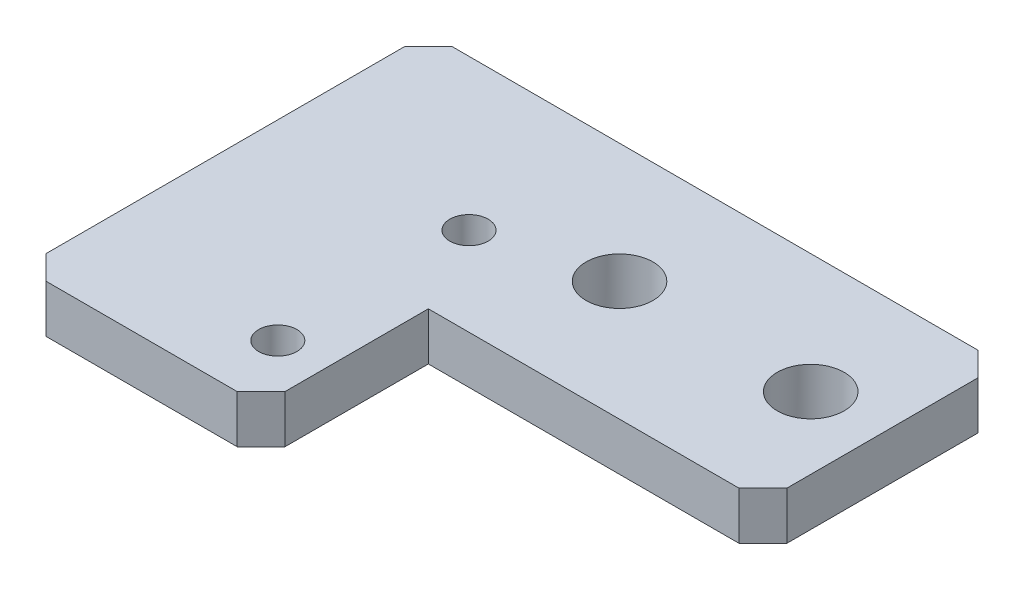
SolidWorks part; units mm, degrees
ref_plane "Front Plane" through (0, 0, 0) normal (0, 0, 1) x (1, 0, 0)
ref_plane "Top Plane" through (0, 0, 0) normal (0, 1, 0) x (1, 0, 0)
ref_plane "Right Plane" through (0, 0, 0) normal (1, 0, 0) x (0, 0, -1)
sketch "Sketch1" plane through (0, 0, 0) normal (0, 1, 0) x (1, 0, 0)
  line L1 (0, 0) -> (10, 0)
  line L2 (0, 0) -> (0, 17)
  line L3 (0, 17) -> (10, 17)
  line L4 (10, 0) -> (10, 17)
  dimension "D1" = 10
  dimension "D2" = 17
extrude "Boss-Extrude1" add sketch "Sketch1" along normal blind 2
sketch "Sketch2" plane through (0, 2, 0) normal (0, 1, 0) x (1, 0, 0)
  line L1 (10, 17) -> (24, 17)
  line L2 (10, 17) -> (10, 7)
  line L3 (10, 7) -> (24, 7)
  line L4 (24, 17) -> (24, 7)
  dimension "D1" = 14
  dimension "D2" = 10
extrude "Boss-Extrude2" add sketch "Sketch2" against normal blind 2
sketch "Sketch3" plane through (0, 2, 0) normal (0, 1, 0) x (1, 0, 0)
  line L0 (24, 12) -> (-49976, 12) construction
  line L1 (24, 7) -> (24, 17) construction
  circle A0 centre (21, 12) radius 1.4
  circle A1 centre (13, 12) radius 1.4
  point P4 (24, 12)
  dimension "D1" = 8
  dimension "D2" = 3
  dimension "D3" = 2.8
extrude "Cut-Extrude1" cut sketch "Sketch3" against normal blind 10
chamfer "Chamfer1" distance 1 angle 45 5 edges at (0, 1, -17) (0, 1, 0) (10, 1, 0) (24, 1, -17) (24, 1, -7)
hole_wizard "M2 Tapped Hole1" positions "Sketch5" profile "Sketch4" tap size "M2" standard "Gb"
sketch "Sketch5" plane through (0, 2, 0) normal (0, 1, 0) x (1, 0, 0)
  point P0 (8, 10.7)
  point P3 (8, 2.7)
sketch "Sketch4" plane through (8, 2, -10.7) normal (1, 0, 0) x (0, 0, 1)
  line L0 (0, 0) -> (0, 5.6807)
  line L1 (0, 5.6807) -> (0.8, 5.2)
  line L2 (0.8, 5.2) -> (0.8, 0)
  line L5 (0.8, 0) -> (0, 0)
  line L10 (0, 5.6807) -> (-0.8, 5.2) construction
  line L11 (0, -6.35) -> (0, 107.95) construction
  dimension "螺纹孔钻头直径" = 1.6
  dimension "螺纹孔钻头深度" = 5.2
  dimension "导头角度" = 118
cosmetic thread "Cosmetic Thread1" parameters "D1"=2.5, "D2"=2
cosmetic thread "Cosmetic Thread2" parameters "D1"=2.5, "D2"=2
